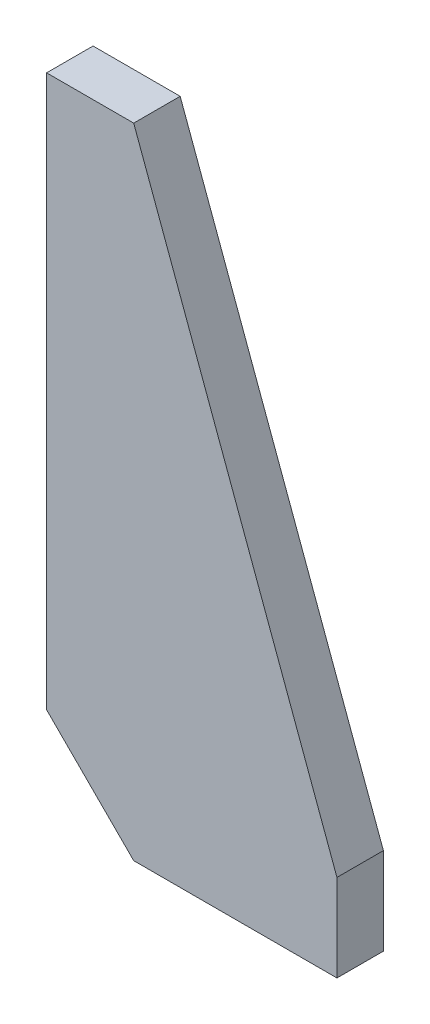
SolidWorks part; units mm, degrees
material "普通碳钢"
ref_plane "Front Plane" through (0, 0, 0) normal (0, 0, 1) x (1, 0, 0)
ref_plane "Top Plane" through (0, 0, 0) normal (0, 1, 0) x (1, 0, 0)
ref_plane "Right Plane" through (0, 0, 0) normal (1, 0, 0) x (0, 0, -1)
sketch "Sketch1" plane through (0, 0, 0) normal (0, 0, 1) x (1, 0, 0)
  line L0 (0, 0) -> (50, 0)
  line L1 (50, 0) -> (50, 15)
  line L2 (50, 15) -> (15, 110)
  line L3 (15, 110) -> (0, 110)
  line L4 (0, 110) -> (0, 0)
  dimension "D1" = 15
  dimension "D2" = 15
  dimension "D3" = 50
  dimension "D4" = 110
extrude "Boss-Extrude1" add sketch "Sketch1" along normal blind 8
chamfer "Chamfer1" distance 15 angle 45 1 edges at (0, 0, 4)
